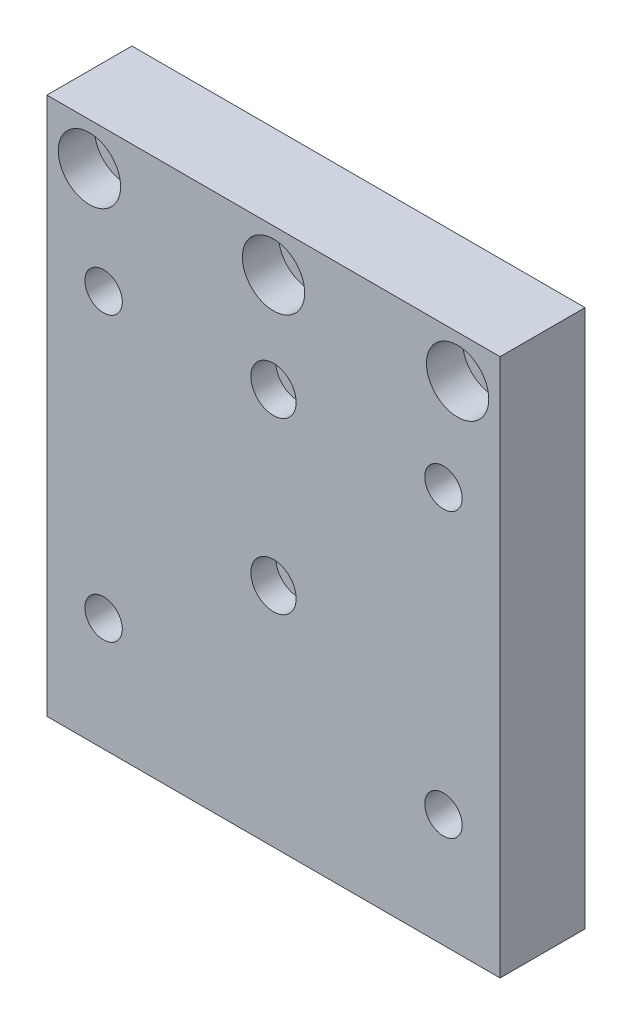
from build123d import *

# Parameters (mm, degrees)
SKETCH_1_W                   = 80
SKETCH_1_H                   = 95
EXTRUDE_1_DEPTH              = 15
HOLE_WIZARD_M4_1_D           = 4.5
HOLE_WIZARD_M4_1_CBORE_D     = 8
HOLE_WIZARD_M4_1_CBORE_DEPTH = 4.4
HOLE_WIZARD_M6_1_D           = 6.6
HOLE_WIZARD_M6_1_CBORE_D     = 11
HOLE_WIZARD_M6_1_CBORE_DEPTH = 6.4
HOLE_WIZARD_M6_2_D           = 6.6
HOLE_WIZARD_M6_2_CBORE_D     = 11
HOLE_WIZARD_M6_2_CBORE_DEPTH = 6.4


with BuildPart() as part:
    # 草图1 → 凸台-拉伸1 (new body)
    with BuildSketch(Plane.XY):
        Rectangle(SKETCH_1_W, SKETCH_1_H)
    extrude(amount=EXTRUDE_1_DEPTH)

    # M4 六角凹头螺钉的柱形沉头孔1 (through all)
    with Locations(Plane.XY.offset(15)):
        with Locations((0, 22.5), (0, -7.5)):
            CounterBoreHole(HOLE_WIZARD_M4_1_D / 2, HOLE_WIZARD_M4_1_CBORE_D / 2, HOLE_WIZARD_M4_1_CBORE_DEPTH)

    # M6 六角凹头螺钉的柱形沉头孔1 (through all)
    with Locations(Plane(origin=(0, 0, 0), x_dir=(-1, 0, 0), z_dir=(0, 0, -1))):
        with Locations((-30, 22.5), (30, 22.5), (30, -27.5), (-30, -27.5)):
            CounterBoreHole(HOLE_WIZARD_M6_1_D / 2, HOLE_WIZARD_M6_1_CBORE_D / 2, HOLE_WIZARD_M6_1_CBORE_DEPTH)

    # M6 六角凹头螺钉的柱形沉头孔2 (through all)
    with Locations(Plane.XY.offset(15)):
        with Locations((-32.5, 40), (0, 40), (32.5, 40)):
            CounterBoreHole(HOLE_WIZARD_M6_2_D / 2, HOLE_WIZARD_M6_2_CBORE_D / 2, HOLE_WIZARD_M6_2_CBORE_DEPTH)


solid = part.part
